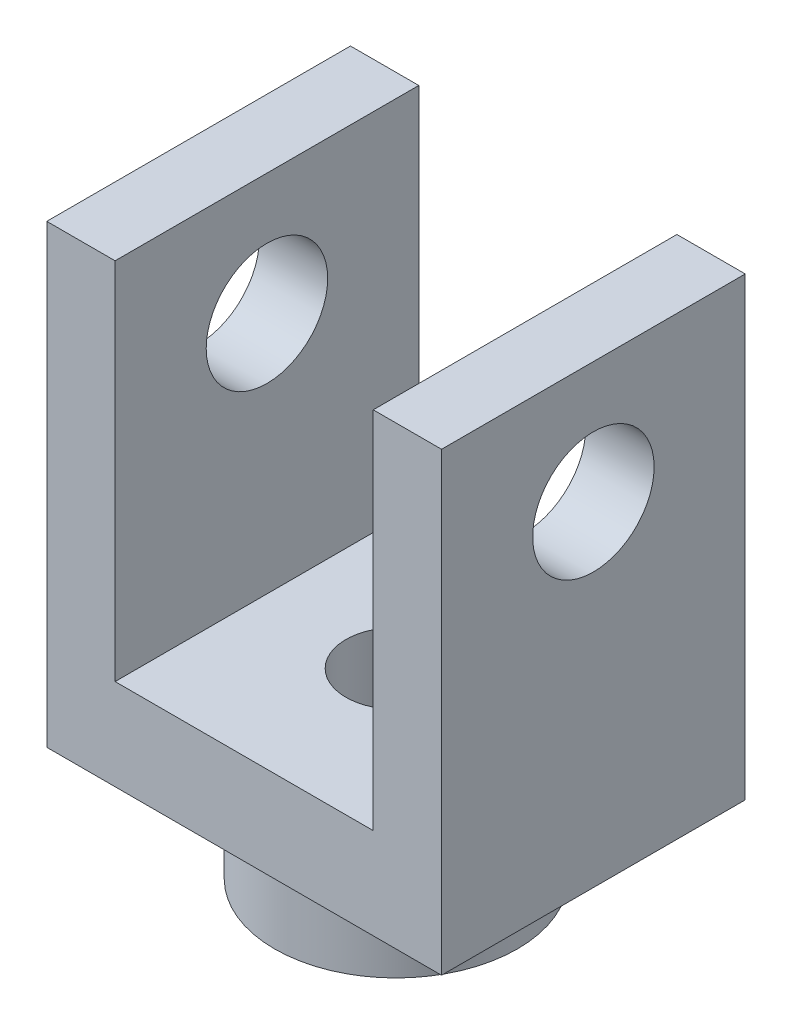
from build123d import *

# Parameters (mm, degrees)
SKETCH_1_W          = 13
SKETCH_1_H          = 15
EXTRUDE_1_DEPTH     = 5
SKETCH_2_W          = 8.5
SKETCH_2_H          = 24
CUT_EXTRUDE_1_DEPTH = 10
SKETCH_3_R          = 2
CUT_EXTRUDE_2_DEPTH = 25
SKETCH_13_R         = 4
EXTRUDE_2_DEPTH     = 3
M4X0_7_1_D          = 3.3
M4X0_7_1_DEPTH      = 10.1
M4X0_7_1_TIP        = 0.991420021


with BuildPart() as part:
    # 草图1 → 凸台-拉伸1 (new, symmetric)
    with BuildSketch(Plane.XY):
        Rectangle(SKETCH_1_W, SKETCH_1_H)
    extrude(amount=EXTRUDE_1_DEPTH, both=True)

    # 草图2 → 切除-拉伸1 (cut)
    with BuildSketch(Plane.XY.offset(5)):
        with Locations((0, 7.5)):
            Rectangle(SKETCH_2_W, SKETCH_2_H)
    extrude(amount=-CUT_EXTRUDE_1_DEPTH, mode=Mode.SUBTRACT)

    # 草图3 → 切除-拉伸2 (cut)
    with BuildSketch(Plane(origin=(6.5, 0, 0), x_dir=(0, 0, -1), z_dir=(1, 0, 0))):
        with Locations((0, 3.5)):
            Circle(SKETCH_3_R)
    extrude(amount=-CUT_EXTRUDE_2_DEPTH, mode=Mode.SUBTRACT)

    # 草图13 → 凸台-拉伸2 (add)
    with BuildSketch(Plane.XZ.offset(7.5)):
        Circle(SKETCH_13_R)
    extrude(amount=EXTRUDE_2_DEPTH)

    # M4x0.7 螺纹孔1
    with Locations(Plane(origin=(0, -10.5, 0), x_dir=(-1, 0, 0), z_dir=(0, -1, 0))):
        with Locations((0, 0)):
            Hole(M4X0_7_1_D / 2, depth=M4X0_7_1_DEPTH)
            with Locations((0, 0, -(M4X0_7_1_DEPTH + M4X0_7_1_TIP / 2))):  # 118° drill point
                Cone(0, M4X0_7_1_D / 2, M4X0_7_1_TIP, mode=Mode.SUBTRACT)


solid = part.part
